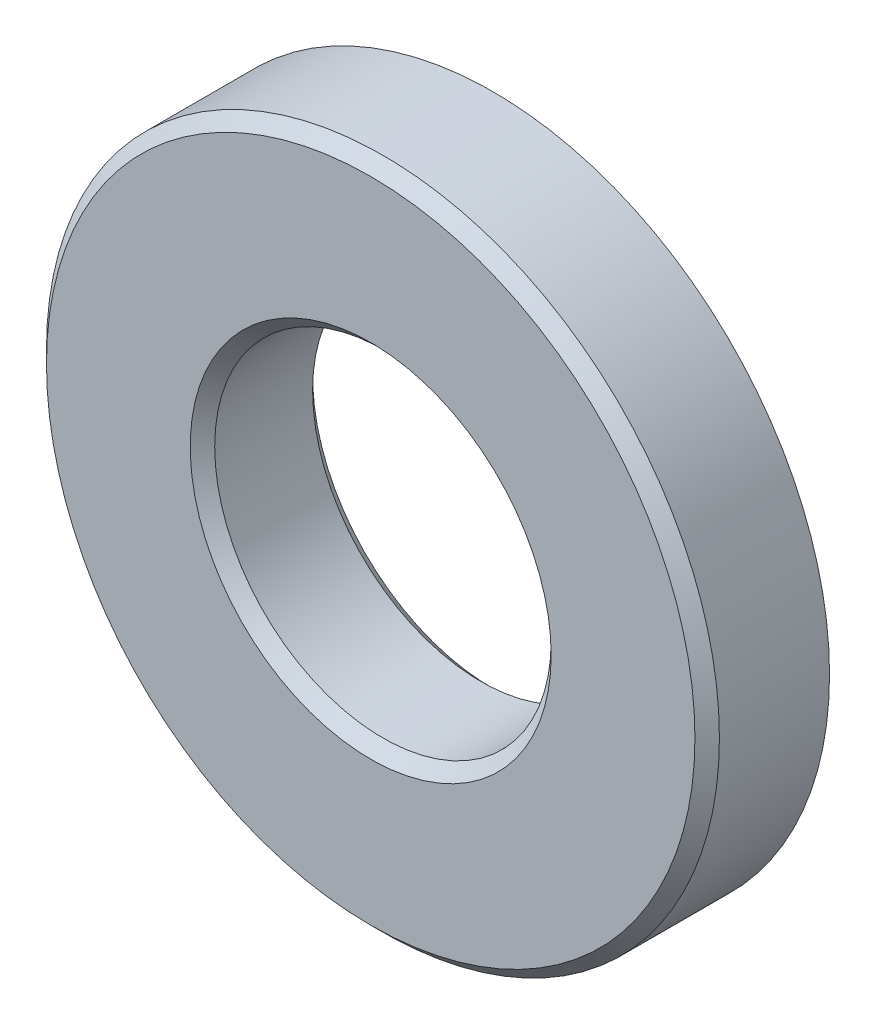
from build123d import *

# Parameters (mm, degrees)
SKETCH1_R           = 55
SKETCH1_R_2         = 27.5
BOSS_EXTRUDE1_DEPTH = 20
CHAMFER1_SIZE       = 2


with BuildPart() as part:
    # Sketch1 → Boss-Extrude1 (new body)
    with BuildSketch(Plane.XY):
        Circle(SKETCH1_R)
        Circle(SKETCH1_R_2, mode=Mode.SUBTRACT)
    extrude(amount=BOSS_EXTRUDE1_DEPTH)

    # Chamfer1
    chamfer1_edges = [part.edges().sort_by_distance(p)[0] for p in [
        (-55, 0, 20),
        (-27.5, 0, 0),
        (-27.5, 0, 20),
    ]]
    chamfer(chamfer1_edges, length=CHAMFER1_SIZE)


solid = part.part
